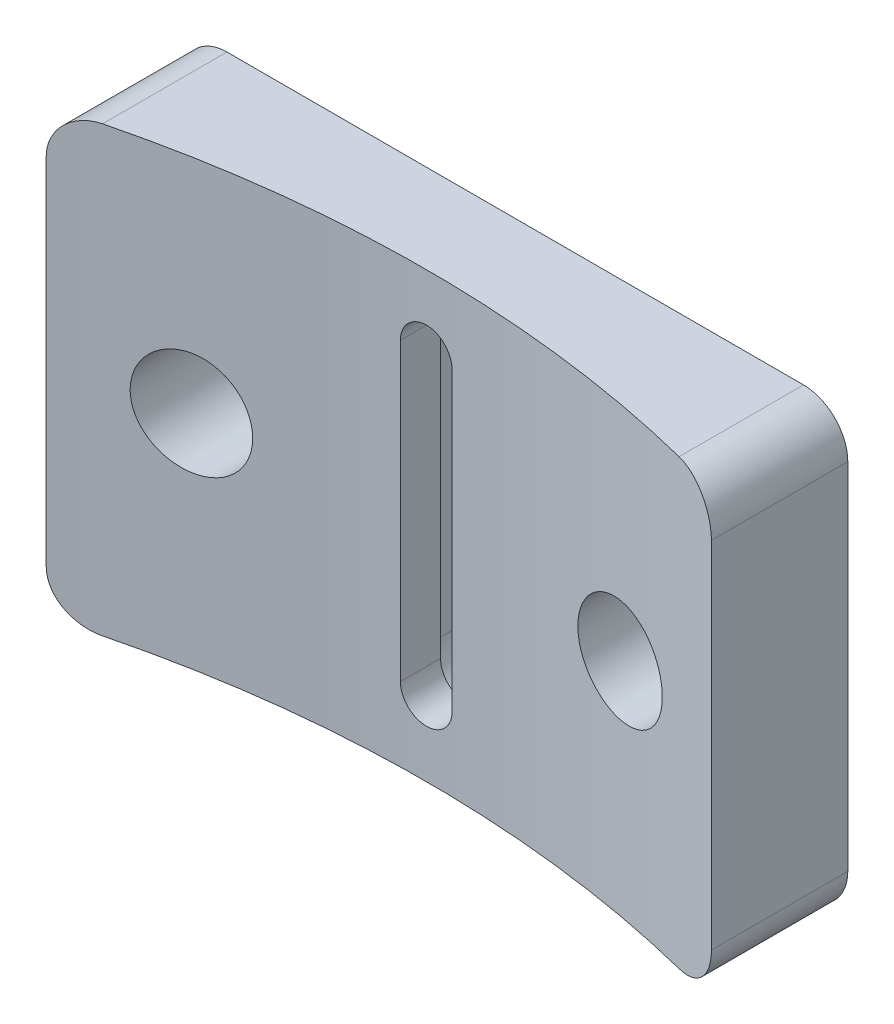
SolidWorks part; units mm, degrees
material "6061-T6 (SS)"
ref_plane "Front Plane" through (0, 0, 0) normal (0, 0, 1) x (1, 0, 0)
ref_plane "Top Plane" through (0, 0, 0) normal (0, 1, 0) x (1, 0, 0)
ref_plane "Right Plane" through (0, 0, 0) normal (1, 0, 0) x (0, 0, -1)
sketch "Sketch1" plane through (0, 0, 0) normal (0, 1, 0) x (1, 0, 0)
  line L0 (-22.5, 76.7708) -> (-22.5, 86)
  line L1 (-22.5, 86) -> (22.5, 86)
  line L2 (22.5, 86) -> (22.5, 76.7708)
  line L3 (0, 0) -> (0, 120.121) construction
  arc A0 (22.5, 76.7708) -> (-22.5, 76.7708) centre (0, 0) ccw
  dimension "D1" = 160
  dimension "D2" = 45
  dimension "D4" = 86
extrude "Boss-Extrude1" add sketch "Sketch1" along normal blind 30
hole_wizard "M8x1.0 Tapped Hole1" positions "Sketch3" profile "Sketch2" tap size "M8x1.0" standard "GB" end condition through all
sketch "Sketch3" plane through (0, 0, -86) normal (0, 0, -1) x (-1, 0, 0)
  line L0 (-22.5, 0) -> (22.5, 0) construction
  line L1 (22.5, 30) -> (-22.5, 30) construction
  line L2 (-22.5, 30) -> (-22.5, 0) construction
  line L3 (22.5, 30) -> (22.5, 0) construction
  point P0 (-14.5, 15)
  point P2 (14.5, 15)
  point P5 (0, 0)
  point P8 (0, 30)
  point P11 (-22.5, 15)
  point P14 (22.5, 15)
  dimension "D1" = 14.5
  dimension "D2" = 14.5
  dimension "D3" = 0
  dimension "D4" = 0
sketch "Sketch2" plane through (14.5, 15, -86) normal (1, 0, 0) x (0, 1, 0)
  line L0 (0, 0) -> (0, 9.2292)
  line L1 (0, 9.2292) -> (3.5, 9.2292)
  line L2 (3.5, 9.2292) -> (3.5, 0)
  line L5 (3.5, 0) -> (0, 0)
  line L11 (0, -6.35) -> (0, 107.95) construction
  dimension "通孔螺纹孔钻头直径" = 7
  dimension "通孔螺纹孔钻头深度" = 9.2292
cosmetic thread "Cosmetic Thread1" parameters "D2"=8
cosmetic thread "Cosmetic Thread2" parameters "D2"=8
sketch "Sketch4" plane through (0, 0, -86) normal (0, 0, -1) x (-1, 0, 0)
  line L0 (0, 0) -> (0, 35.1081) construction
  line L2 (-22.5, 15) -> (24.5658, 15) construction
  line L3 (-22.5, 30) -> (-22.5, 0) construction
  line L5 (0, 25) -> (0, 5) construction
  line L6 (1.75, 25) -> (1.75, 5)
  line L7 (-1.75, 25) -> (-1.75, 5)
  arc A2 (1.75, 25) -> (-1.75, 25) centre (0, 25) ccw
  arc A3 (-1.75, 5) -> (1.75, 5) centre (0, 5) ccw
  point P15 (0, 15)
  dimension "D6" = 1.75
  dimension "D5" = 20
extrude "Cut-Extrude1" cut sketch "Sketch4" against normal through all
sketch "Sketch5" plane through (0, 0, -86) normal (0, 0, -1) x (-1, 0, 0)
  line L0 (0, 25) -> (0, 5) construction
  line L1 (3, 25) -> (3, 5)
  line L2 (-3, 25) -> (-3, 5)
  arc A0 (3, 25) -> (-3, 25) centre (0, 25) ccw
  arc A1 (-3, 5) -> (3, 5) centre (0, 5) ccw
  point P2 (0, 15)
  dimension "D1" = 3
extrude "Cut-Extrude2" cut sketch "Sketch5" against normal blind 3.3
fillet "Fillet1" radius 3 4 edges at (-22.5, 30, -81.3854) (22.5, 30, -81.3854) (-22.5, 0, -81.3854) (22.5, 0, -81.3854)
